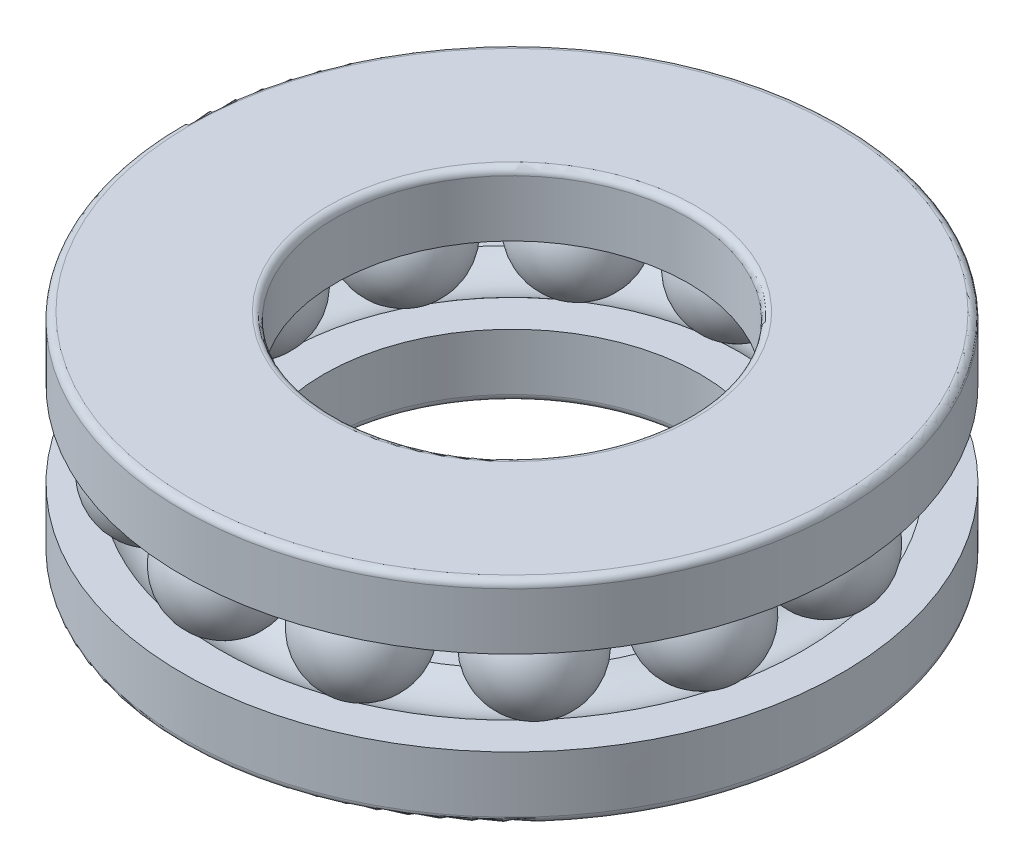
SolidWorks part; units mm, degrees
ref_plane "Plane1" through (0, 0, 0) normal (0, 0, 1) x (1, 0, 0)
ref_plane "Plane2" through (0, 0, 0) normal (0, 1, 0) x (1, 0, 0)
ref_plane "Plane3" through (0, 0, 0) normal (1, 0, 0) x (0, 0, -1)
sketch "Dimension Sketch" plane through (0, 0, 0) normal (0, 0, 1) x (1, 0, 0)
  line L0 (0, 0) -> (28, 0)
  point P3 (15, 0)
  point P4 (16, 0)
  point P5 (28, 0)
  point P6 (9, 0)
  point P7 (0.3, 0)
sketch "Sketch1" plane through (0, 0, 0) normal (0, 0, 1) x (1, 0, 0)
  line L0 (14, 0) -> (14, 30.489) construction
  line L1 (0, 0) -> (28, 0)
  line L2 (0, 0) -> (0, 9)
  line L3 (0, 9) -> (28, 9)
  line L4 (28, 0) -> (28, 9)
  line L5 (6.5, 0) -> (6.5, 58.489)
  line L6 (21.5, 0) -> (21.5, 58.489)
  line L7 (0, 0) -> (0, 58.489)
  line L8 (28, 0) -> (28, 58.489)
  line L9 (6, 0) -> (6, 58.489)
  line L10 (22, 0) -> (22, 58.489)
  line L11 (0, 4.5) -> (28, 4.5) construction
  line L12 (25, 0) -> (25, 58.489)
  line L13 (3, 0) -> (3, 58.489)
  line L14 (0, 2.7) -> (250, 2.7)
  line L15 (0, 6.3) -> (250, 6.3)
  circle A0 centre (3, 4.5) radius 2.25
sketch "Sketch2" plane through (0, 0, 0) normal (0, 0, 1) x (1, 0, 0)
  line L0 (0, 2.7) -> (250, 2.7) construction
  line L1 (14, 0) -> (14, 30.489) construction
  line L2 (6, 0) -> (6, 58.489) construction
  line L3 (0, 2.7) -> (1.65, 2.7)
  line L4 (0, 0) -> (28, 0)
  line L5 (28, 0) -> (28, 9)
  line L6 (28, 9) -> (0, 9)
  line L7 (0, 9) -> (0, 0)
  line L8 (0, 0) -> (6, 0)
  line L9 (4.35, 2.7) -> (6, 2.7)
  line L11 (0, 2.7) -> (0, 0)
  line L12 (14, 0) -> (14, 30.489) construction
  line L13 (6, 0) -> (6, 2.7)
  circle A0 centre (3, 4.5) radius 2.25 construction
  arc A1 (1.65, 2.7) -> (4.35, 2.7) centre (3, 4.5) ccw
  dimension "D1" = 0
revolve "Base-Revolve" add sketch "Sketch2" angle 360 about L12
sketch "Sketch3" plane through (0, 0, 0) normal (0, 0, 1) x (1, 0, 0)
  line L2 (3, 0) -> (3, 58.489) construction
  line L3 (3, 0) -> (3, 58.489) construction
  line L4 (3, 2.2) -> (3, 6.8)
  circle A0 centre (3, 4.5) radius 2.25 construction
  arc A1 (3, 6.75) -> (3, 2.25) centre (3, 4.5) ccw construction
  arc A2 (3, 6.8) -> (3, 2.2) centre (3, 4.5) ccw
  dimension "D1" = 0.05
revolve "Boss-Revolve2" add sketch "Sketch3" angle 360 about L3
sketch "Sketch4" plane through (0, 0, 0) normal (0, 0, 1) x (1, 0, 0)
  line L0 (14, 0) -> (14, 30.489) construction
  line L1 (0, 6.3) -> (250, 6.3) construction
  line L2 (6.5, 0) -> (6.5, 58.489) construction
  line L3 (0, 0) -> (0, 58.489) construction
  line L4 (0, 9) -> (28, 9) construction
  line L5 (14, 0) -> (14, 30.489) construction
  line L6 (0, 6.3) -> (1.65, 6.3)
  line L7 (6.5, 6.3) -> (6.5, 9)
  line L8 (0, 6.3) -> (0, 9)
  line L9 (0, 9) -> (6.5, 9)
  line L12 (4.35, 6.3) -> (6.5, 6.3)
  circle A0 centre (3, 4.5) radius 2.25 construction
  arc A1 (4.35, 6.3) -> (1.65, 6.3) centre (3, 4.5) ccw
revolve "Boss-Revolve3" add sketch "Sketch4" angle 360 about L5
pattern_circular "CirPattern1" count 13 over 360 about axis through (14, 0, 0) along (0, 1, 0) of "Boss-Revolve2"
fillet "Fillet1" radius 0.3 4 edges at (14, 9, -7.5) (14, 9, -14) (14, 0, -8) (14, 0, -14)
equation "\"D1@Sketch1\" = \"DD@Dimension Sketch\""
equation "\"D5@Sketch1\" = \"d1@Dimension Sketch\""
equation "\"D4@Sketch1\" = \"d@Dimension Sketch\""
equation "\"D3@Sketch1\" = \"DD1@Dimension Sketch\""
equation "\"D2@Sketch1\" = \"T@Dimension Sketch\""
equation "\"D1@Fillet1\" = \"r@Dimension Sketch\""
equation "\"D6@Sketch1\" =  ( \"D5@Sketch1\" + \"D1@Sketch1\" )  / 2"
equation "\"D7@Sketch1\" = \"D2@Sketch1\" * 0.4"
equation "\"D8@Sketch1\" = \"D2@Sketch1\" / 2"
equation "\"D1@CirPattern1\" = 3.14*(\"D1@Sketch1\" + \"D5@Sketch1\" )  / 2 / \"D8@Sketch1\"*0.85"
